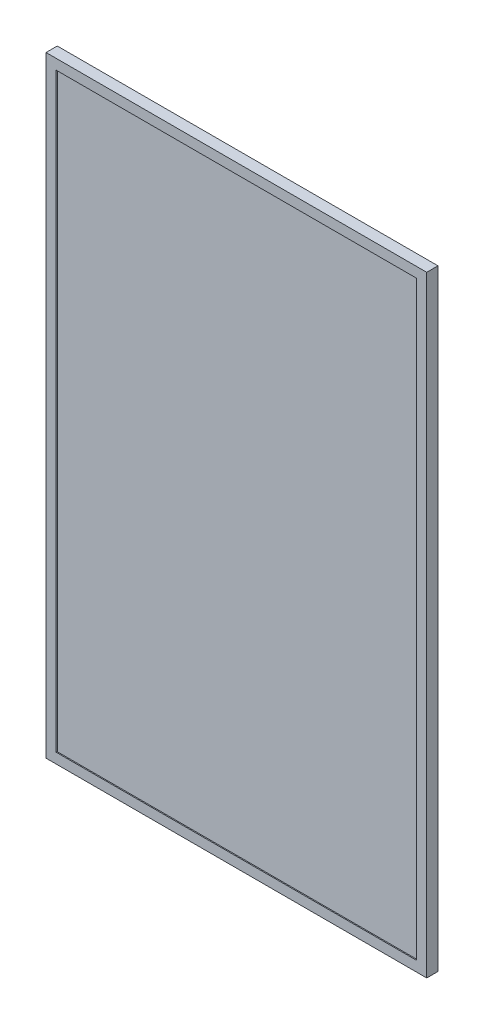
SolidWorks part; units mm, degrees
ref_plane "前视基准面" through (0, 0, 0) normal (0, 0, 1) x (1, 0, 0)
ref_plane "上视基准面" through (0, 0, 0) normal (0, 1, 0) x (1, 0, 0)
ref_plane "右视基准面" through (0, 0, 0) normal (1, 0, 0) x (0, 0, -1)
sketch "草图1" plane through (0, 0, 0) normal (0, 0, 1) x (1, 0, 0)
  line L1 (0, 0) -> (745, 0)
  line L2 (0, 0) -> (0, 1196)
  line L3 (0, 1196) -> (745, 1196)
  line L4 (745, 0) -> (745, 1196)
  dimension "D1" = 1196
  dimension "D2" = 745
extrude "凸台-拉伸1" add sketch "草图1" along normal blind 22
shell "抽壳1" thickness 2
sketch "草图2" plane through (0, 0, 22) normal (0, 0, 1) x (1, 0, 0)
  line L14 (20, 1176) -> (20, 20)
  line L15 (20, 20) -> (725, 20)
  line L16 (725, 20) -> (725, 1176)
  line L17 (725, 1176) -> (20, 1176)
  line L18 (20, 1176) -> (20, 20)
  line L19 (20, 20) -> (725, 20)
  line L20 (725, 20) -> (725, 1176)
  line L21 (725, 1176) -> (20, 1176)
  line L26 (0, 1196) -> (0, 0)
  line L27 (0, 0) -> (745, 0)
  line L28 (745, 0) -> (745, 1196)
  line L29 (745, 1196) -> (0, 1196)
  line L30 (0, 1196) -> (0, 0)
  line L31 (0, 0) -> (745, 0)
  line L32 (745, 0) -> (745, 1196)
  line L33 (745, 1196) -> (0, 1196)
  dimension "D1" = 20
  dimension "D2" = 0
extrude "凸台-拉伸2" add sketch "草图2" against normal blind 2
